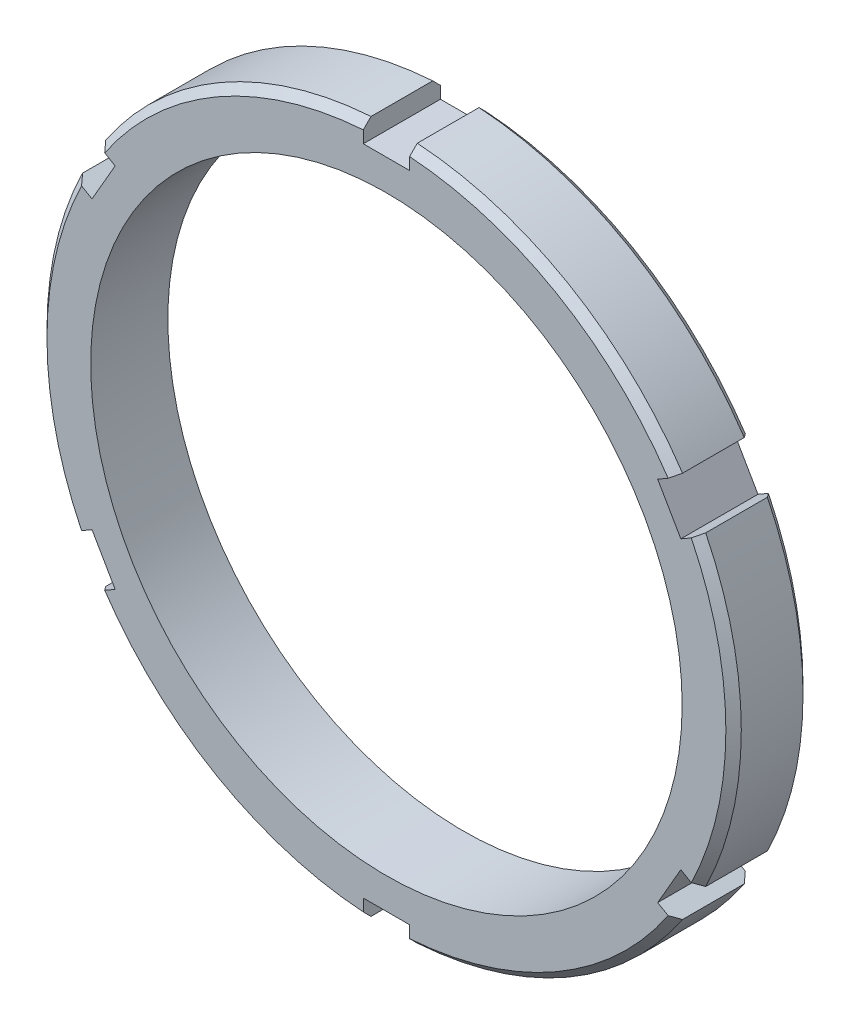
SolidWorks part; units mm, degrees
material "45"
ref_plane "Front Plane" through (0, 0, 0) normal (0, 0, 1) x (1, 0, 0)
ref_plane "Top Plane" through (0, 0, 0) normal (0, 1, 0) x (1, 0, 0)
ref_plane "Right Plane" through (0, 0, 0) normal (1, 0, 0) x (0, 0, -1)
sketch "Sketch1" plane through (0, 0, 0) normal (1, 0, 0) x (0, 0, -1)
  line L0 (0, 0) -> (135.2434, 0) construction
  line L1 (0, 0) -> (0, 143.1757) construction
  line L2 (0, 135) -> (30, 135)
  line L3 (30, 135) -> (30, 115)
  line L4 (30, 115) -> (0, 115)
  line L5 (0, 115) -> (0, 135)
  dimension "D1" = 115
  dimension "D2" = 135
  dimension "D3" = 30
revolve "Revolve1" add sketch "Sketch1" angle 360 about L0
chamfer "Chamfer1" distance 3 angle 45 2 edges at (135, 0, -30) (135, 0, 0)
sketch "Sketch2" plane through (0, 0, 0) normal (0, 0, 1) x (1, 0, 0)
  line L0 (0, 0) -> (0, 151.3897) construction
  line L1 (9, 127) -> (-9, 127)
  line L2 (9, 127) -> (9, 143)
  line L3 (9, 143) -> (-9, 143)
  line L4 (-9, 127) -> (-9, 143)
  line L5 (9, 127) -> (-9, 143) construction
  line L6 (9, 143) -> (-9, 127) construction
  circle A0 centre (0, 0) radius 135 construction
  point P0 (0, 135)
  dimension "D1" = 18
  dimension "D2" = 8
extrude "Cut-Extrude1" cut sketch "Sketch2" against normal blind 38
pattern_circular "CirPattern1" count 6 over 360 about axis through (0, 0, 0) along (0, 0, 1) of "Cut-Extrude1"
